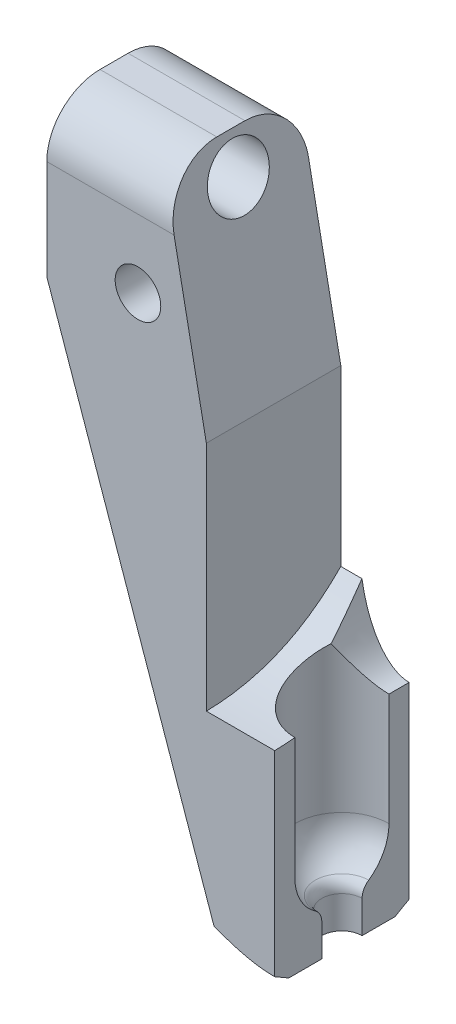
from build123d import *

# Parameters (mm, degrees)
SKETCH1_R                      = 3
BOSS_EXTRUDE2_DEPTH            = 17.7
CUT_EXTRUDE1_REACH             = 94.786
CUT_EXTRUDE1_DIRECTION_2_REACH = 94.786
SKETCH6_RX                     = 12.258033
SKETCH6_RY                     = 6.491927
CUT_EXTRUDE2_DEPTH             = 48.7
SKETCH7_R                      = 6.19409
CUT_EXTRUDE3_DEPTH             = 60.7
SKETCH8_R                      = 4
CUT_EXTRUDE4_DEPTH             = 48
FILLET1_R                      = 7
SKETCH10_OUTSIDE_W             = 249.546
SKETCH10_OUTSIDE_H             = 207.246
SKETCH10_OUTSIDE_R             = 7
CUT_EXTRUDE5_DEPTH             = 48
CUT_EXTRUDE5_TAPER             = 60
CUT_EXTRUDE7_DEPTH             = 44


with BuildPart() as part:
    # Sketch1 → Boss-Extrude2 (new body)
    with BuildSketch(Plane.XY):
        with BuildLine():
            Line((39, -51.503555), (34.837666, -51.503555))
            Line((34.837666, -51.503555), (25.162334, -51.503555))
            Line((25.162334, -51.503555), (21, -51.503555))
            Line((21, -51.503555), (21, -28.6))
            Line((21, -28.6), (15.376404, 0))
            Line((15.376404, 0), (0, 0))
            Line((0, 0), (0, -20.136364))
            Line((0, -20.136364), (21.048788, -80.412439))
            add(Edge.make_bspline(
                [(21.669142, -82.188906), (21.466678, -81.609123), (21.259066, -81.014599), (21.048788, -80.412439)],
                knots=[0.75, 0.75, 0.75, 0.75, 1, 1, 1, 1], degree=3))
            add(Edge.make_bspline(
                [(22.255532, -83.868113), (22.06924, -83.334643), (21.871606, -82.768689), (21.669142, -82.188906)],
                knots=[0.5, 0.5, 0.5, 0.5, 0.75, 0.75, 0.75, 0.75], degree=3))
            add(Edge.make_bspline(
                [(22.524034, -84.637007), (22.439154, -84.393941), (22.348677, -84.134848), (22.255532, -83.868113)],
                knots=[0.375, 0.375, 0.375, 0.375, 0.5, 0.5, 0.5, 0.5], degree=3))
            add(Edge.make_bspline(
                [(22.758263, -85.307753), (22.688292, -85.107381), (22.608914, -84.880073), (22.524034, -84.637007)],
                knots=[0.25, 0.25, 0.25, 0.25, 0.375, 0.375, 0.375, 0.375], degree=3))
            add(Edge.make_bspline(
                [(22.855261, -85.585519), (22.825847, -85.50129), (22.793248, -85.407938), (22.758263, -85.307753)],
                knots=[0.1875, 0.1875, 0.1875, 0.1875, 0.25, 0.25, 0.25, 0.25], degree=3))
            add(Edge.make_bspline(
                [(22.932474, -85.806631), (22.910958, -85.745015), (22.884674, -85.669748), (22.855261, -85.585519)],
                knots=[0.125, 0.125, 0.125, 0.125, 0.1875, 0.1875, 0.1875, 0.1875], degree=3))
            add(Edge.make_bspline(
                [(23, -86), (22.975508, -85.929864), (22.932474, -85.806631)],
                knots=[0, 0, 0, 0.125, 0.125, 0.125], degree=2))
            Line((23, -86), (37, -86))
            add(Edge.make_bspline(
                [(37.068167, -85.804796), (37.025162, -85.927946), (37, -86)],
                knots=[0.875, 0.875, 0.875, 1, 1, 1], degree=2))
            add(Edge.make_bspline(
                [(37.242328, -85.306061), (37.171936, -85.507639), (37.111171, -85.681646), (37.068167, -85.804796)],
                knots=[0.75, 0.75, 0.75, 0.75, 0.875, 0.875, 0.875, 0.875], degree=3))
            add(Edge.make_bspline(
                [(37.47673, -84.63482), (37.392157, -84.877005), (37.31272, -85.104482), (37.242328, -85.306061)],
                knots=[0.625, 0.625, 0.625, 0.625, 0.75, 0.75, 0.75, 0.75], degree=3))
            add(Edge.make_bspline(
                [(37.744144, -83.869041), (37.651111, -84.135454), (37.561302, -84.392634), (37.47673, -84.63482)],
                knots=[0.5, 0.5, 0.5, 0.5, 0.625, 0.625, 0.625, 0.625], degree=3))
            add(Edge.make_bspline(
                [(38.330881, -82.18884), (38.128355, -82.768803), (37.930211, -83.336215), (37.744144, -83.869041)],
                knots=[0.25, 0.25, 0.25, 0.25, 0.5, 0.5, 0.5, 0.5], degree=3))
            add(Edge.make_bspline(
                [(38.951212, -80.412439), (38.741, -81.014409), (38.533408, -81.608878), (38.330881, -82.18884)],
                knots=[0, 0, 0, 0, 0.25, 0.25, 0.25, 0.25], degree=3))
            Line((38.951212, -80.412439), (60, -20.136364))
            Line((60, -20.136364), (60, 0))
            Line((60, 0), (44.6, 0))
            Line((44.6, 0), (39, -28))
            Line((39, -28), (39, -51.503555))
        make_face()
        with Locations((48, -16)):
            Circle(SKETCH1_R, mode=Mode.SUBTRACT)
        with Locations((12, -16)):
            Circle(SKETCH1_R, mode=Mode.SUBTRACT)
    extrude(amount=BOSS_EXTRUDE2_DEPTH)

    # Sketch2 → Cut-Revolve2 (revolve, cut)
    with BuildSketch(Plane.ZY.offset(-30), mode=Mode.PRIVATE) as cut_revolve2_sk:
        with BuildLine():
            ThreePointArc((11.5, -81.75), (11.729241, -80.820262), (12.364412, -80.103659))
            ThreePointArc((12.364412, -80.103659), (14.333443, -77.882187), (15.04409, -75))
            Line((15.04409, -75), (15.04409, -57.48))
            Line((15.04409, -57.48), (8.85, -57.48))
            Line((8.85, -57.48), (8.85, -86))
            Line((8.85, -86), (11.5, -86))
            Line((11.5, -86), (11.5, -81.75))
        make_face()
    revolve(cut_revolve2_sk.sketch.rotate(Axis((30, -86, 8.85), (0, 1, 0)), 180), axis=Axis((30, -86, 8.85), (0, 1, 0)), mode=Mode.SUBTRACT)

    # Cut-Extrude1: up to this face of the body (flat: up to its plane)
    cut_extrude1_end = Plane(part.part.faces().sort_by_distance((39, -39.751777, 8.85))[0])
    # Sketch3 → Cut-Extrude1 (cut, up to the picked face)
    with BuildSketch(Plane.ZY.offset(-30), mode=Mode.PRIVATE) as cut_extrude1_sk1:
        with BuildLine():
            Line((0, -51.503555), (17.7, -51.503555))
            Line((17.7, -51.503555), (17.7, -59.152297))
            add(Edge.make_bspline(
                [(17.7, -59.152297), (7.335394, -59.008853), (0, -51.503555)],
                knots=[0, 0, 0, 1, 1, 1], degree=2))
        make_face()
    cut_extrude1_tool1 = split(extrude(cut_extrude1_sk1.sketch, amount=-CUT_EXTRUDE1_REACH, mode=Mode.PRIVATE), bisect_by=cut_extrude1_end, keep=Keep.BOTH, mode=Mode.PRIVATE)
    add(cut_extrude1_tool1.solids().sort_by(Axis((30, -54.604638, 10.907898), (1, 0, 0)))[0], mode=Mode.SUBTRACT)

    # Cut-Extrude1 direction 2: up to this face of the body (flat: up to its plane)
    cut_extrude1_direction_2_end = Plane(part.part.faces().sort_by_distance((21, -40.051777, 8.85))[0])
    # Sketch3 → Cut-Extrude1 direction 2 (cut, up to the picked face)
    with BuildSketch(Plane.ZY.offset(-30), mode=Mode.PRIVATE) as cut_extrude1_direction_2_sk1:
        with BuildLine():
            Line((0, -51.503555), (17.7, -51.503555))
            Line((17.7, -51.503555), (17.7, -59.152297))
            add(Edge.make_bspline(
                [(17.7, -59.152297), (7.335394, -59.008853), (0, -51.503555)],
                knots=[0, 0, 0, 1, 1, 1], degree=2))
        make_face()
    cut_extrude1_direction_2_tool1 = split(extrude(cut_extrude1_direction_2_sk1.sketch, amount=CUT_EXTRUDE1_DIRECTION_2_REACH, mode=Mode.PRIVATE), bisect_by=cut_extrude1_direction_2_end, keep=Keep.BOTH, mode=Mode.PRIVATE)
    add(cut_extrude1_direction_2_tool1.solids().sort_by(Axis((30, -54.604638, 10.907898), (-1, 0, 0)))[0], mode=Mode.SUBTRACT)

    # Sketch6 → Cut-Extrude2 (cut)
    with BuildSketch(Plane(origin=(0, 0, 8.85), x_dir=(-1, 0, 0), z_dir=(0, 0, -1))):
        with Locations(Location((-30, -47.968312), (0, 0, 90))):
            Ellipse(SKETCH6_RX, SKETCH6_RY)
    extrude(amount=CUT_EXTRUDE2_DEPTH, mode=Mode.SUBTRACT)

    # Sketch7 → Cut-Extrude3 (cut)
    with BuildSketch(Plane(origin=(0, 0, 0), x_dir=(1, 0, 0), z_dir=(0, 1, 0))):
        with Locations(Location((30, -8.85, 0), (0, 0, 90))):
            Circle(SKETCH7_R)
    extrude(amount=-CUT_EXTRUDE3_DEPTH, mode=Mode.SUBTRACT)

    # Sketch8 → Cut-Extrude4 (cut)
    with BuildSketch(Plane.ZY.offset(-6)):
        with Locations((8.85, -5)):
            Circle(SKETCH8_R)
    extrude(amount=-CUT_EXTRUDE4_DEPTH, mode=Mode.SUBTRACT)

    # Fillet1
    fillet1_edges = [part.edges().sort_by_distance(p)[0] for p in [
        (7.688202, 0, 17.7),
        (52.3, 0, 0),
        (7.688202, 0, 0),
        (52.3, 0, 17.7),
    ]]
    fillet(fillet1_edges, radius=FILLET1_R)

    # Sketch10 outside → Cut-Extrude5 (cut)
    with BuildSketch(Plane.XZ.offset(86)):
        with Locations((30, 8.85)):
            Rectangle(SKETCH10_OUTSIDE_W, SKETCH10_OUTSIDE_H)
        with Locations((30, 8.85)):
            Circle(SKETCH10_OUTSIDE_R, mode=Mode.SUBTRACT)
    extrude(amount=-CUT_EXTRUDE5_DEPTH, taper=CUT_EXTRUDE5_TAPER, mode=Mode.SUBTRACT)

    # Sketch12 → Cut-Extrude7 (cut)
    with BuildSketch(Plane.XY.offset(17.7)):
        Polygon((30, -86), (30, 13.730719), (80.816645, 10.061019), (70.681282, -110.340096), align=None)
    extrude(amount=-CUT_EXTRUDE7_DEPTH, mode=Mode.SUBTRACT)


solid = part.part
